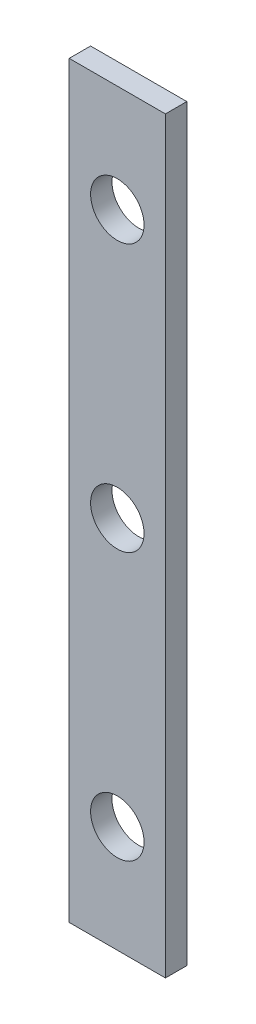
SolidWorks part; units mm, degrees
material "Q235B"
ref_plane "Front Plane" through (0, 0, 0) normal (0, 0, 1) x (1, 0, 0)
ref_plane "Top Plane" through (0, 0, 0) normal (0, 1, 0) x (1, 0, 0)
ref_plane "Right Plane" through (0, 0, 0) normal (1, 0, 0) x (0, 0, -1)
other "Configuration Table"
sketch "Sketch 1" plane through (0, 0, 0) normal (0, 0, 1) x (1, 0, 0)
  line L1 (-9, -70) -> (9, -70)
  line L2 (-9, -70) -> (-9, 70)
  line L3 (-9, 70) -> (9, 70)
  line L4 (9, -70) -> (9, 70)
  line L5 (-9, -70) -> (9, 70) construction
  line L6 (-9, 70) -> (9, -70) construction
  circle A0 centre (0, 50) radius 5
  circle A1 centre (0, 0) radius 5
  circle A2 centre (0, -50) radius 5
  point P0 (0, 0)
  dimension "D5" = 10
  dimension "D1" = 18
  dimension "D2" = 140
  dimension "D3" = 100
  dimension "D4" = 50
extrude "Boss-Extrude1" add sketch "Sketch 1" along normal blind 4
